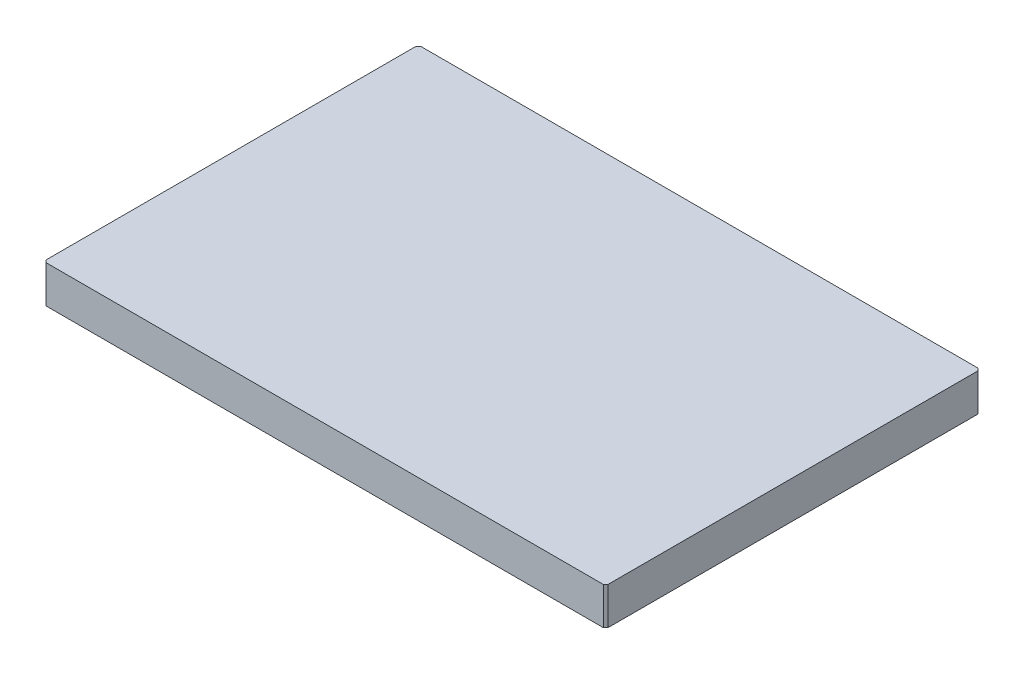
SolidWorks part; units mm, degrees
ref_plane "Front Plane" through (0, 0, 0) normal (0, 0, 1) x (1, 0, 0)
ref_plane "Top Plane" through (0, 0, 0) normal (0, 1, 0) x (1, 0, 0)
ref_plane "Right Plane" through (0, 0, 0) normal (1, 0, 0) x (0, 0, -1)
sketch "Sketch1" plane through (0, 0, 0) normal (0, 1, 0) x (1, 0, 0)
  line L1 (-600, 400) -> (600, 400)
  line L2 (-600, 400) -> (-600, -400)
  line L3 (-600, -400) -> (600, -400)
  line L4 (600, 400) -> (600, -400)
  line L5 (-600, 400) -> (600, -400) construction
  line L6 (-600, -400) -> (600, 400) construction
  point P0 (0, 0)
  dimension "D1" = 1200
  dimension "D2" = 800
extrude "Boss-Extrude1" add sketch "Sketch1" along normal blind 80
chamfer "Chamfer1" distance 5 angle 45 4 edges at (600, 40, -400) (-600, 40, -400) (600, 40, 400) (-600, 40, 400)
hole_wizard "M16 Tapped Hole1" positions "Sketch2" profile "Sketch3" tap size "M16" standard "ISO"
sketch "Sketch2" plane through (0, 0, 0) normal (0, -1, 0) x (-1, 0, 0)
  point P0 (0, -200)
  point P3 (100, -173.2051)
  point P6 (173.2051, -100)
  point P9 (200, 0)
  point P12 (173.2051, 100)
  point P15 (100, 173.2051)
  point P18 (0, 200)
  point P21 (-100, 173.2051)
  point P24 (-173.2051, 100)
  point P27 (-200, 0)
  point P30 (-173.2051, -100)
  point P33 (-100, -173.2051)
sketch "Sketch3" plane through (0, 0, 200) normal (1, 0, 0) x (0, 0, -1)
  line L0 (0, 0) -> (0, 42.206)
  line L1 (0, 42.206) -> (7, 38)
  line L2 (7, 38) -> (7, 0)
  line L5 (7, 0) -> (0, 0)
  line L10 (0, 42.206) -> (-7, 38) construction
  line L11 (0, -6.35) -> (0, 107.95) construction
  dimension "螺纹孔钻头直径" = 14
  dimension "螺纹孔钻头深度" = 38
  dimension "导头角度" = 118
cosmetic thread "Cosmetic Thread1"
cosmetic thread "Cosmetic Thread2"
cosmetic thread "Cosmetic Thread3"
cosmetic thread "Cosmetic Thread4"
cosmetic thread "Cosmetic Thread5"
cosmetic thread "Cosmetic Thread6"
cosmetic thread "Cosmetic Thread7"
cosmetic thread "Cosmetic Thread8"
cosmetic thread "Cosmetic Thread9"
cosmetic thread "Cosmetic Thread10"
cosmetic thread "Cosmetic Thread11"
cosmetic thread "Cosmetic Thread12"
